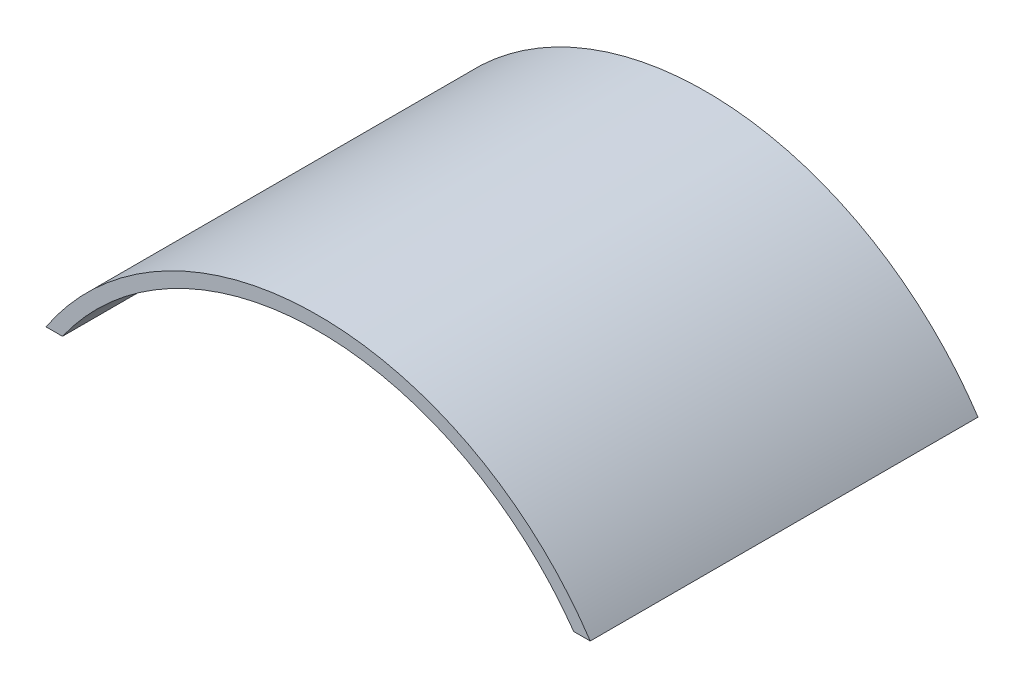
from build123d import *

# Parameters (mm, degrees)
BOSS_EXTRUDE1_DEPTH = 28.5


with BuildPart() as part:
    # Sketch1 → Boss-Extrude1 (new, symmetric)
    with BuildSketch(Plane.XY):
        with BuildLine():
            Line((-40, 26.532998323), (-37.576588456, 26.532998323))
            ThreePointArc((-37.576588456, 26.532998323), (0, 46), (37.576588456, 26.532998323))
            Line((37.576588456, 26.532998323), (40, 26.532998323))
            ThreePointArc((40, 26.532998323), (0, 48), (-40, 26.532998323))
        make_face()
    extrude(amount=BOSS_EXTRUDE1_DEPTH, both=True)


solid = part.part
